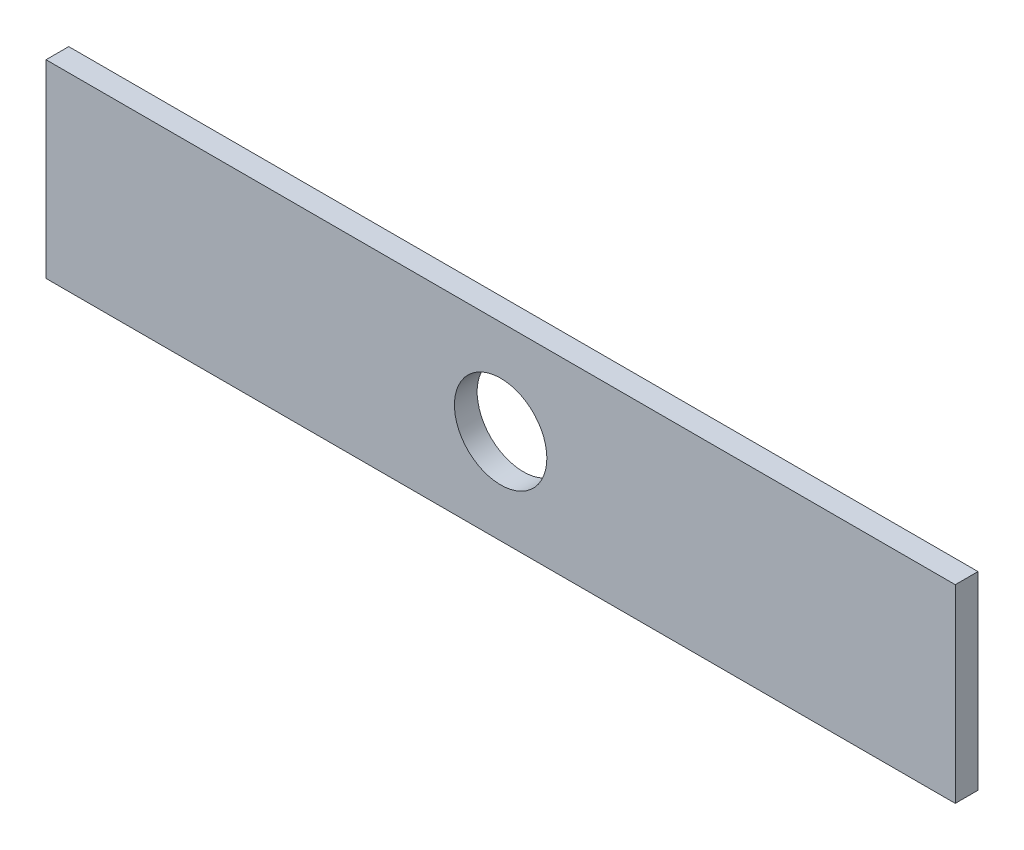
from build123d import *

# Parameters (mm, degrees)
SKETCH_1_W          = 120
SKETCH_1_H          = 25
EXTRUDE_1_DEPTH     = 1.5
SKETCH_2_R          = 6.1
CUT_EXTRUDE_1_DEPTH = 11.5


with BuildPart() as part:
    # 草图1 → 凸台-拉伸1 (new, symmetric)
    with BuildSketch(Plane.XY):
        Rectangle(SKETCH_1_W, SKETCH_1_H)
    extrude(amount=EXTRUDE_1_DEPTH, both=True)

    # 草图2 → 切除-拉伸1 (cut, symmetric)
    with BuildSketch(Plane.XY):
        Circle(SKETCH_2_R)
    extrude(amount=CUT_EXTRUDE_1_DEPTH, both=True, mode=Mode.SUBTRACT)


solid = part.part
